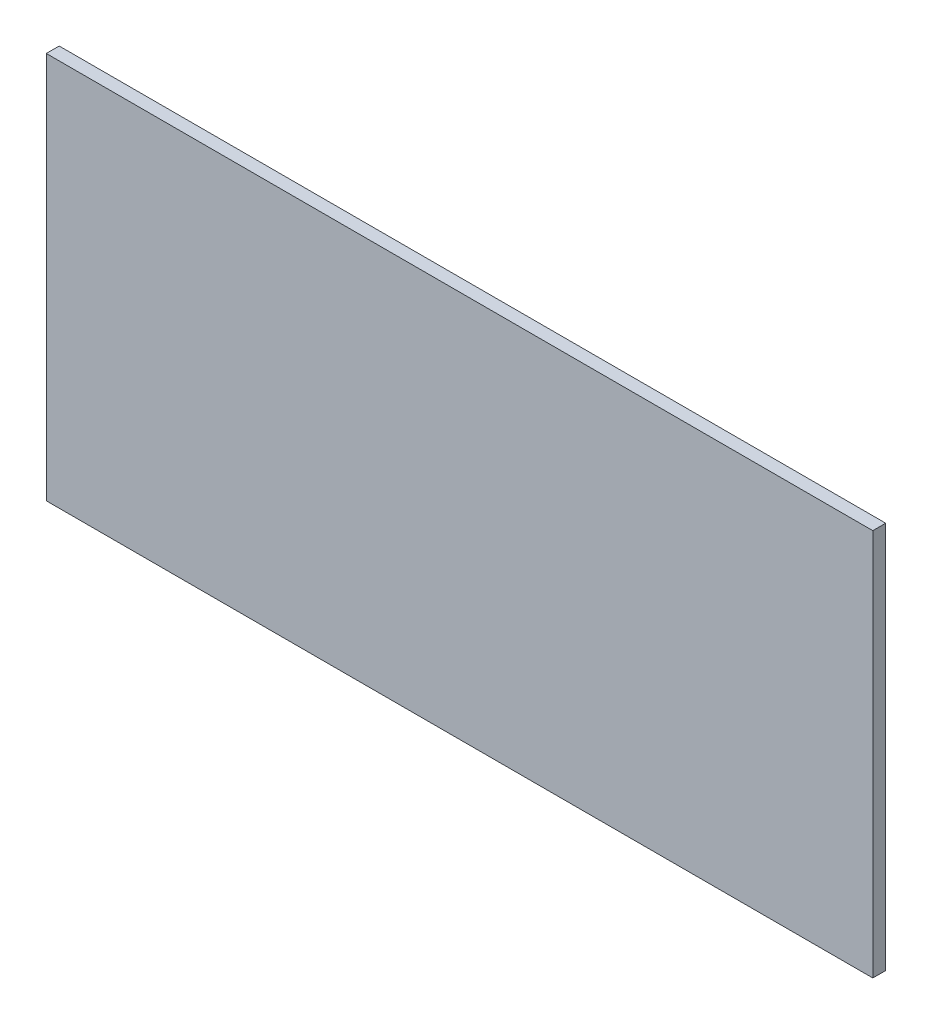
from build123d import *

# Parameters (mm, degrees)
SKETCH1_W           = 640
SKETCH1_H           = 300
BOSS_EXTRUDE1_DEPTH = 10


with BuildPart() as part:
    # Sketch1 → Boss-Extrude1 (new body)
    with BuildSketch(Plane.XY):
        with Locations((320, 150)):
            Rectangle(SKETCH1_W, SKETCH1_H)
    extrude(amount=BOSS_EXTRUDE1_DEPTH)


solid = part.part
